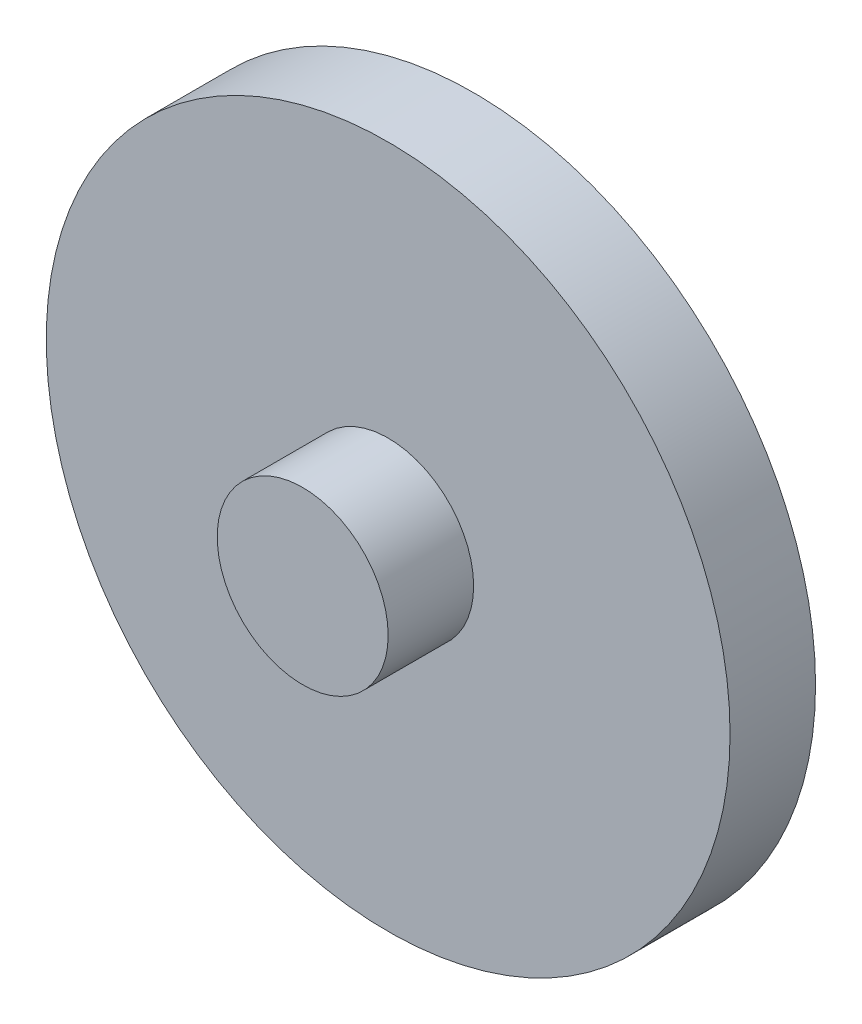
from build123d import *

# Parameters (mm, degrees)
SKETCH_1_R      = 40
EXTRUDE_1_DEPTH = 10
SKETCH_2_R      = 10
EXTRUDE_2_DEPTH = 20


with BuildPart() as part:
    # 草图1 → 凸台-拉伸1 (new body)
    with BuildSketch(Plane.XY):
        Circle(SKETCH_1_R)
    extrude(amount=EXTRUDE_1_DEPTH)

    # 草图2 → 凸台-拉伸2 (add)
    with BuildSketch(Plane.XY):
        Circle(SKETCH_2_R)
    extrude(amount=EXTRUDE_2_DEPTH)


solid = part.part
